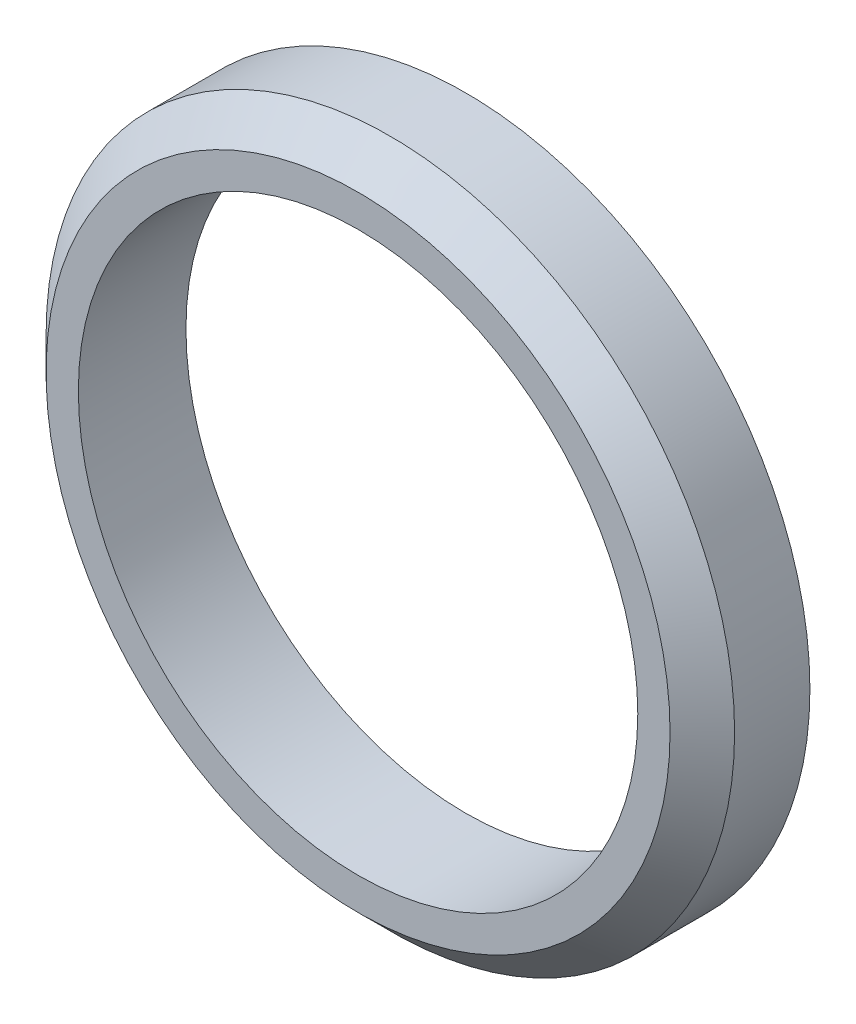
from build123d import *

# Parameters (mm, degrees)
SKETCH1_R           = 16
SKETCH1_R_2         = 13
BOSS_EXTRUDE1_DEPTH = 5
CHAMFER1_SIZE       = 1.5


with BuildPart() as part:
    # Sketch1 → Boss-Extrude1 (new body)
    with BuildSketch(Plane.XY):
        Circle(SKETCH1_R)
        Circle(SKETCH1_R_2, mode=Mode.SUBTRACT)
    extrude(amount=BOSS_EXTRUDE1_DEPTH)

    # Chamfer1
    chamfer1_edges = [part.edges().sort_by_distance(p)[0] for p in [
        (-16, 0, 5),
    ]]
    chamfer(chamfer1_edges, length=CHAMFER1_SIZE)


solid = part.part
